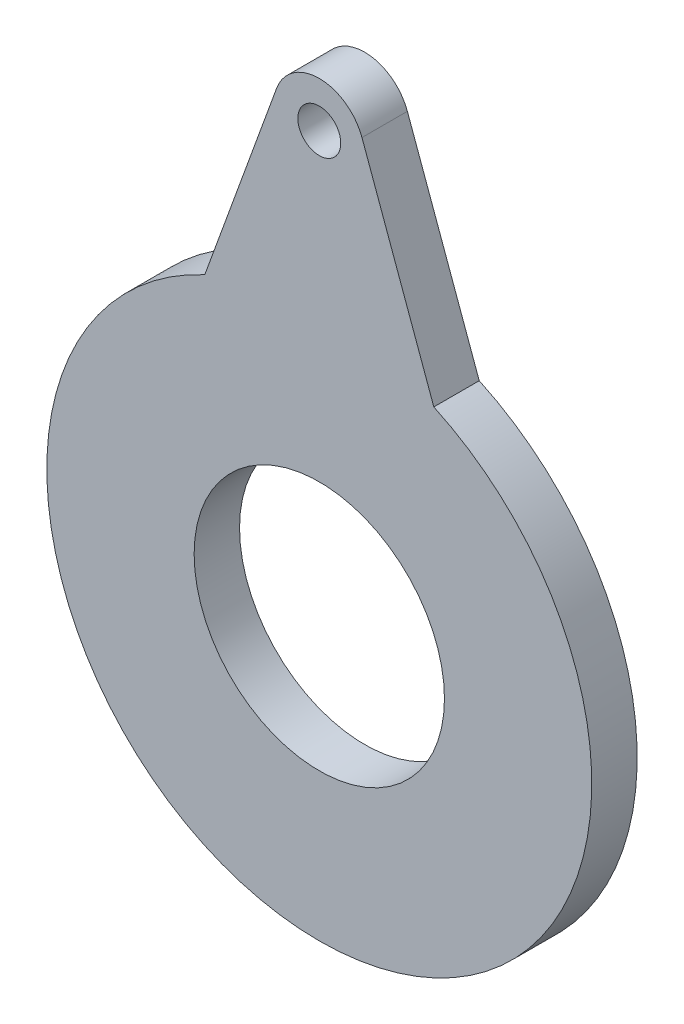
from build123d import *

# Parameters (mm, degrees)
SKETCH1_R           = 26.2509
SKETCH1_R_2         = 4.5
BOSS_EXTRUDE1_DEPTH = 9.525


with BuildPart() as part:
    # Sketch1 → Boss-Extrude1 (new body)
    with BuildSketch(Plane.XY.offset(222.25)):
        with BuildLine():
            Line((-8.950572213, 93.257741865), (-24.018992106, 51.857598462))
            ThreePointArc((-24.018992106, 51.857598462), (0, -57.15), (24.018992106, 51.857598462))
            Line((24.018992106, 51.857598462), (8.950572213, 93.257741865))
            ThreePointArc((8.950572213, 93.257741865), (0, 99.525), (-8.950572213, 93.257741865))
        make_face()
        with Locations(Location((0, 0, 0), (0, 0, 180))):
            Circle(SKETCH1_R, mode=Mode.SUBTRACT)
        with Locations(Location((0, 90, 0), (0, 0, 180))):
            Circle(SKETCH1_R_2, mode=Mode.SUBTRACT)
    extrude(amount=BOSS_EXTRUDE1_DEPTH)


solid = part.part
